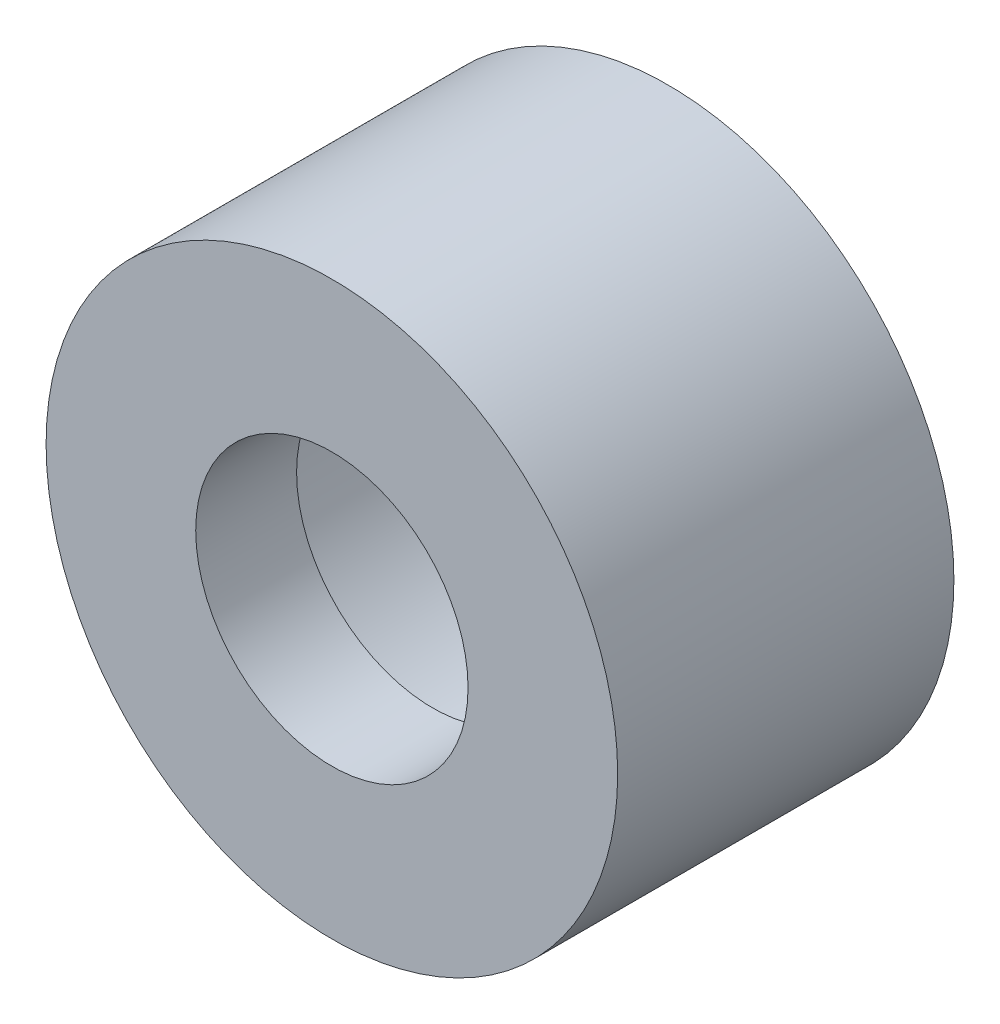
from build123d import *

# Parameters (mm, degrees)
SKETCH_1_R          = 8.5
SKETCH_1_R_2        = 4.05
EXTRUDE_1_DEPTH     = 10
SKETCH_2_R          = 6.25
CUT_EXTRUDE_1_DEPTH = 7


with BuildPart() as part:
    # 草图1 → 凸台-拉伸1 (new body)
    with BuildSketch(Plane.XY):
        Circle(SKETCH_1_R)
        Circle(SKETCH_1_R_2, mode=Mode.SUBTRACT)
    extrude(amount=EXTRUDE_1_DEPTH)

    # 草图2 → 切除-拉伸1 (cut)
    with BuildSketch(Plane(origin=(0, 0, 0), x_dir=(-1, 0, 0), z_dir=(0, 0, -1))):
        Circle(SKETCH_2_R)
    extrude(amount=-CUT_EXTRUDE_1_DEPTH, mode=Mode.SUBTRACT)


solid = part.part
